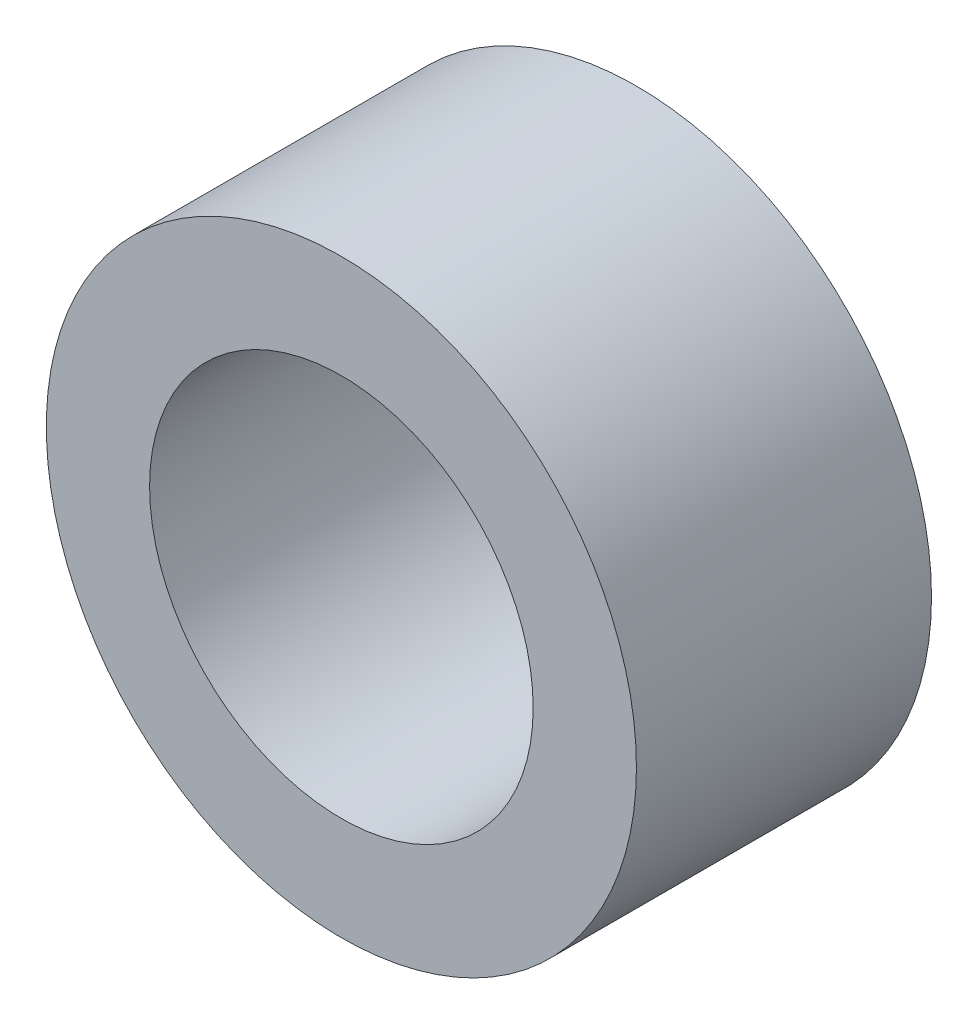
from build123d import *

# Parameters (mm, degrees)
SKETCH1_R          = 10
EXTRUDE1_DEPTH     = 10
SKETCH2_R          = 6.5
CUT_EXTRUDE1_DEPTH = 10


with BuildPart() as part:
    # Sketch1 → Extrude1 (new body)
    with BuildSketch(Plane.XY):
        Circle(SKETCH1_R)
    extrude(amount=EXTRUDE1_DEPTH)

    # Sketch2 → Cut-Extrude1 (cut)
    with BuildSketch(Plane.XY.offset(10)):
        Circle(SKETCH2_R)
    extrude(amount=-CUT_EXTRUDE1_DEPTH, mode=Mode.SUBTRACT)


solid = part.part
